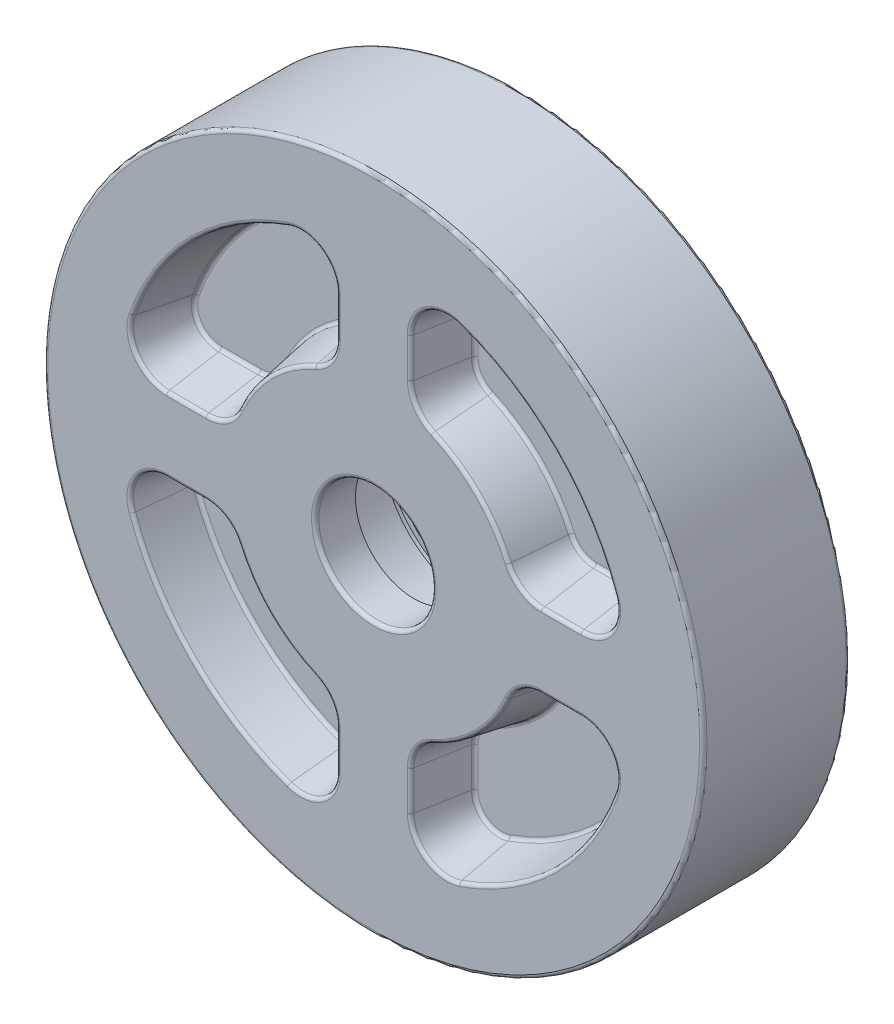
SolidWorks part; units mm, degrees
ref_plane "Front Plane" through (0, 0, 0) normal (0, 0, 1) x (1, 0, 0)
ref_plane "Top Plane" through (0, 0, 0) normal (0, 1, 0) x (1, 0, 0)
ref_plane "Right Plane" through (0, 0, 0) normal (1, 0, 0) x (0, 0, -1)
sketch "Sketch1" plane through (0, 0, 0) normal (0, 0, 1) x (1, 0, 0)
  circle A0 centre (0, 0) radius 90
  dimension "D1" = 180
extrude "Boss-Extrude1" add sketch "Sketch1" along normal mid plane 40
sketch "Sketch2" plane through (0, 0, 20) normal (0, 0, 1) x (1, 0, 0)
  circle A0 centre (0, 0) radius 16
  dimension "D1" = 32
extrude "Cut-Extrude1" cut sketch "Sketch2" against normal blind 11
sketch "Sketch3" plane through (0, 0, 9) normal (0, 0, 1) x (1, 0, 0)
  circle A0 centre (0, 0) radius 22.5
  dimension "D1" = 45
extrude "Cut-Extrude2" cut sketch "Sketch3" against normal blind 2
sketch "Sketch4" plane through (0, 0, 7) normal (0, 0, 1) x (1, 0, 0)
  circle A0 centre (0, 0) radius 26
  dimension "D1" = 52
extrude "Cut-Extrude3" cut sketch "Sketch4" against normal blind 15
sketch "Sketch5" plane through (0, 0, -8) normal (0, 0, 1) x (1, 0, 0)
  circle A0 centre (0, 0) radius 27.5
  dimension "D1" = 55
extrude "Cut-Extrude4" cut sketch "Sketch5" against normal blind 2
sketch "Sketch6" plane through (0, 0, -10) normal (0, 0, 1) x (1, 0, 0)
  circle A0 centre (0, 0) radius 26
  dimension "D1" = 52
extrude "Cut-Extrude5" cut sketch "Sketch6" against normal through all
sketch "Sketch7" plane through (0, 0, -20) normal (0, 0, -1) x (-1, 0, 0)
  line L1 (-10, 56.5685) -> (-10, 45.8258)
  line L7 (-56.5685, 10) -> (-45.8258, 10)
  arc A0 (-16, 36.6606) -> (-36.6606, 16) centre (0, 0) ccw
  arc A1 (-23.3333, 65.9966) -> (-65.9966, 23.3333) centre (0, 0) ccw
  arc A2 (-65.9966, 23.3333) -> (-56.5685, 10) centre (-56.5685, 20) ccw
  arc A3 (-45.8258, 10) -> (-36.6606, 16) centre (-45.8258, 20) ccw
  arc A4 (-10, 45.8258) -> (-16, 36.6606) centre (-20, 45.8258) cw
  arc A5 (-10, 56.5685) -> (-23.3333, 65.9966) centre (-20, 56.5685) ccw
  point P4 (0, 77.2067)
  point P5 (0, 31.6517)
  point P6 (-10, 77.2067)
  point P7 (-10, 31.6517)
  point P8 (10, 77.2067)
  point P9 (10, 31.6517)
  point P28 (0, 0)
  dimension "D1" = 80
  dimension "D2" = 140
  dimension "D3" = 10
extrude "Cut-Extrude6" cut sketch "Sketch7" against normal blind 15 draft 10
pattern_circular "CirPattern1" count 4 over 360 about axis through (0, 0, 0) along (0, 0, 1) of "Cut-Extrude6"
mirror "Mirror1" about plane through (0, 0, 0) normal (0, 0, 1) of "CirPattern1", "Cut-Extrude6"
fillet "Fillet1" radius 1 66 edges at (51.1971, 12.6449, 5) (41.7972, 13.8463, 5) (30.1545, 30.1545, 5) (13.8463, 41.7972, 5) (12.6449, 51.1971, 5) (15.7535, 62.574, 5) (47.6272, 47.6272, 5) (62.574, 15.7535, 5) (12.6449, -51.1971, 5) (13.8463, -41.7972, 5) (30.1545, -30.1545, 5) (41.7972, -13.8463, 5) (51.1971, -12.6449, 5) (62.574, -15.7535, 5) (47.6272, -47.6272, 5) (15.7535, -62.574, 5) (-51.1971, -12.6449, 5) (-41.7972, -13.8463, 5) (-30.1545, -30.1545, 5) (-13.8463, -41.7972, 5) (-12.6449, -51.1971, 5) (-15.7535, -62.574, 5) (-47.6272, -47.6272, 5) (-62.574, -15.7535, 5) (-12.6449, 51.1971, 5) (-13.8463, 41.7972, 5) (-30.1545, 30.1545, 5) (-41.7972, 13.8463, 5) (-51.1971, 12.6449, 5) (-62.574, 15.7535, 5) (-47.6272, 47.6272, 5) (-15.7535, 62.574, 5) (-64.7335, 14.2265, 20) (-51.1971, 10, 20) (-40.3485, 11.6334, 20) (-28.2843, 28.2843, 20) (-11.6334, 40.3485, 20) (-10, 51.1971, 20) (-14.2265, 64.7335, 20) (-49.4975, 49.4975, 20) (64.7335, -14.2265, 20) (51.1971, -10, 20) (40.3485, -11.6334, 20) (28.2843, -28.2843, 20) (11.6334, -40.3485, 20) (10, -51.1971, 20) (14.2265, -64.7335, 20) (49.4975, -49.4975, 20) (90, 0, 20) (16, 0, 20) (14.2265, 64.7335, 20) (10, 51.1971, 20) (11.6334, 40.3485, 20) (28.2843, 28.2843, 20) (40.3485, 11.6334, 20) (51.1971, 10, 20) (64.7335, 14.2265, 20) (49.4975, 49.4975, 20) (-14.2265, -64.7335, 20) (-10, -51.1971, 20) (-11.6334, -40.3485, 20) (-28.2843, -28.2843, 20) (-40.3485, -11.6334, 20) (-51.1971, -10, 20) (-64.7335, -14.2265, 20) (-49.4975, -49.4975, 20)
fillet "Fillet2" radius 1 66 edges at (47.6272, 47.6272, -5) (15.7535, 62.574, -5) (12.6449, 51.1971, -5) (13.8463, 41.7972, -5) (30.1545, 30.1545, -5) (41.7972, 13.8463, -5) (51.1971, 12.6449, -5) (62.574, 15.7535, -5) (47.6272, -47.6272, -5) (62.574, -15.7535, -5) (51.1971, -12.6449, -5) (41.7972, -13.8463, -5) (30.1545, -30.1545, -5) (13.8463, -41.7972, -5) (12.6449, -51.1971, -5) (15.7535, -62.574, -5) (-47.6272, -47.6272, -5) (-15.7535, -62.574, -5) (-12.6449, -51.1971, -5) (-13.8463, -41.7972, -5) (-30.1545, -30.1545, -5) (-41.7972, -13.8463, -5) (-51.1971, -12.6449, -5) (-62.574, -15.7535, -5) (-47.6272, 47.6272, -5) (-62.574, 15.7535, -5) (-51.1971, 12.6449, -5) (-41.7972, 13.8463, -5) (-30.1545, 30.1545, -5) (-13.8463, 41.7972, -5) (-12.6449, 51.1971, -5) (-15.7535, 62.574, -5) (90, 0, -20) (26, 0, -20) (40.3485, 11.6334, -20) (28.2843, 28.2843, -20) (11.6334, 40.3485, -20) (10, 51.1971, -20) (14.2265, 64.7335, -20) (49.4975, 49.4975, -20) (64.7335, 14.2265, -20) (51.1971, 10, -20) (11.6334, -40.3485, -20) (28.2843, -28.2843, -20) (40.3485, -11.6334, -20) (51.1971, -10, -20) (64.7335, -14.2265, -20) (49.4975, -49.4975, -20) (14.2265, -64.7335, -20) (10, -51.1971, -20) (-40.3485, -11.6334, -20) (-28.2843, -28.2843, -20) (-11.6334, -40.3485, -20) (-10, -51.1971, -20) (-14.2265, -64.7335, -20) (-49.4975, -49.4975, -20) (-64.7335, -14.2265, -20) (-51.1971, -10, -20) (-11.6334, 40.3485, -20) (-28.2843, 28.2843, -20) (-40.3485, 11.6334, -20) (-51.1971, 10, -20) (-64.7335, 14.2265, -20) (-49.4975, 49.4975, -20) (-14.2265, 64.7335, -20) (-10, 51.1971, -20)
sketch "Sketch8" plane through (0, 0, -20) normal (0, 0, -1) x (-1, 0, 0)
  circle A1 centre (0, 32.5) radius 1.5
  circle A2 centre (28.1458, -16.25) radius 1.5
  circle A3 centre (-28.1458, -16.25) radius 1.5
  point P12 (0, 0)
  dimension "D1" = 3
  dimension "D3" = 3
extrude "Cut-Extrude7" cut sketch "Sketch8" against normal blind 10
